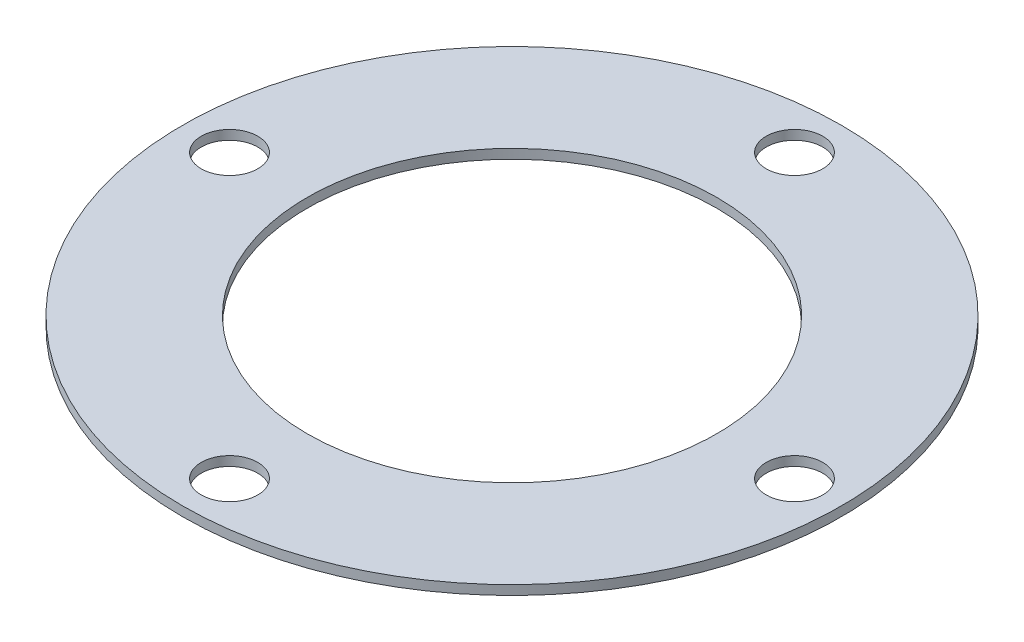
from build123d import *

# Parameters (mm, degrees)
SKETCH_1_R          = 70
SKETCH_1_R_2        = 43.5
EXTRUDE_1_DEPTH     = 2
SKETCH_3_R          = 6
CUT_EXTRUDE_1_DEPTH = 100.015150356


with BuildPart() as part:
    # 草图1 → 凸台-拉伸1 (new body)
    with BuildSketch(Plane(origin=(0, 0, 0), x_dir=(1, 0, 0), z_dir=(0, 1, 0))):
        with Locations(Location((0, 0, 0), (0, 0, 270))):
            Circle(SKETCH_1_R)
        with Locations(Location((0, 0, 0), (0, 0, 270))):
            Circle(SKETCH_1_R_2, mode=Mode.SUBTRACT)
    extrude(amount=EXTRUDE_1_DEPTH)

    # 草图3 → 切除-拉伸1 (cut, through all)
    with BuildSketch(Plane(origin=(0, 2, 0), x_dir=(1, 0, 0), z_dir=(0, 1, 0))):
        with Locations(Location((0, 60, 0), (0, 0, 270))):
            Circle(SKETCH_3_R)
        with Locations(Location((60, 0, 0), (0, 0, 270))):
            Circle(SKETCH_3_R)
        with Locations(Location((0, -60, 0), (0, 0, 270))):
            Circle(SKETCH_3_R)
        with Locations(Location((-60, 0, 0), (0, 0, 270))):
            Circle(SKETCH_3_R)
    extrude(amount=-CUT_EXTRUDE_1_DEPTH, mode=Mode.SUBTRACT)


solid = part.part
